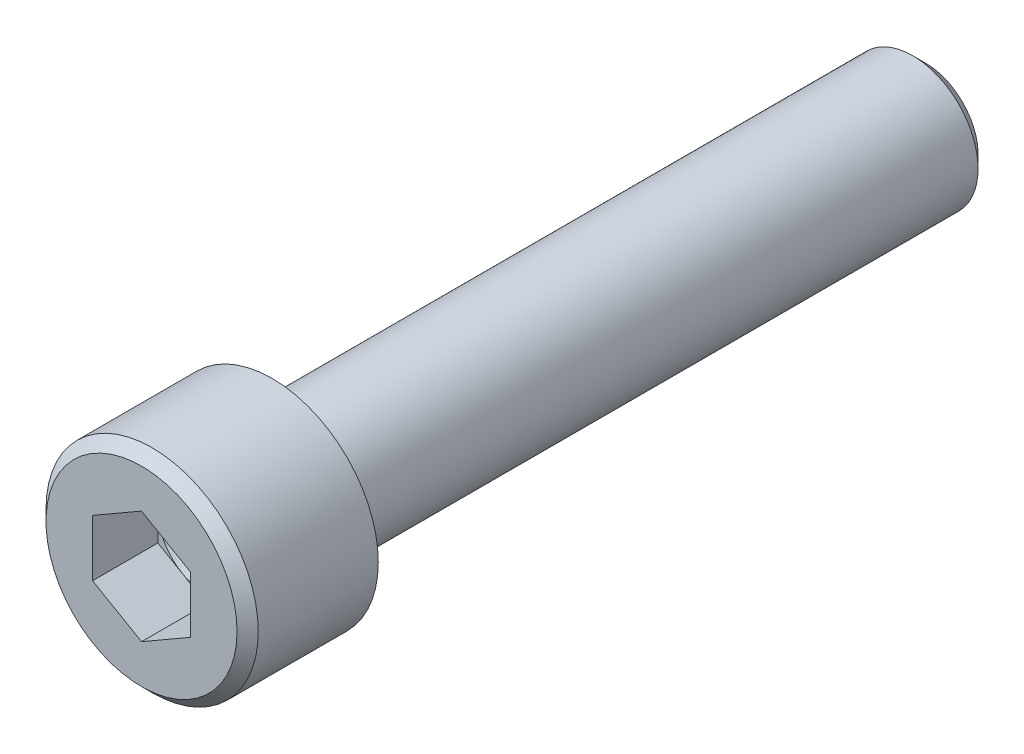
from build123d import *

# Parameters (mm, degrees)
SKETCH_1_W          = 6.5
SKETCH_1_H          = 8
SKETCH_2_R          = 4
EXTRUDE_1_DEPTH     = 40
CUT_EXTRUDE_1_DEPTH = 4
CHAMFER_1_SIZE      = 0.65
CHAMFER_2_SIZE      = 0.767


with BuildPart() as part:
    # 草图1 → 旋转1 (revolve)
    with BuildSketch(Plane(origin=(0, 0, 0), x_dir=(1, 0, 0), z_dir=(0, 1, 0))):
        with Locations((3.25, -4)):
            Rectangle(SKETCH_1_W, SKETCH_1_H)
    revolve(axis=Axis((0, 0, 0), (0, 0, 1)))

    # 草图2 → 凸台-拉伸1 (add)
    with BuildSketch(Plane(origin=(0, 0, 0), x_dir=(-1, 0, 0), z_dir=(0, 0, -1))):
        Circle(SKETCH_2_R)
    extrude(amount=EXTRUDE_1_DEPTH)

    # 草图3 → 切除-拉伸1 (cut)
    with BuildSketch(Plane.XY.offset(8)):
        Polygon((3, 1.732050808), (0, 3.464101615), (-3, 1.732050808), (-3, -1.732050808), (0, -3.464101615), (3, -1.732050808), align=None)
    extrude(amount=-CUT_EXTRUDE_1_DEPTH, mode=Mode.SUBTRACT)

    # 草图4 → 切除-旋转1 (revolve, cut)
    with BuildSketch(Plane.XZ, mode=Mode.PRIVATE) as cut_revolve_1_sk:
        Polygon((3, 4), (0, 4), (0, 2.267949192), align=None)
    revolve(cut_revolve_1_sk.sketch.rotate(Axis((0, 0, 4), (0, 0, -1)), 90), axis=Axis((0, 0, 4), (0, 0, -1)), mode=Mode.SUBTRACT)

    # 倒角1
    chamfer_1_edges = [part.edges().sort_by_distance(p)[0] for p in [
        (-6.5, 0, 8),
    ]]
    chamfer(chamfer_1_edges, length=CHAMFER_1_SIZE)

    # 倒角2
    chamfer_2_edges = [part.edges().sort_by_distance(p)[0] for p in [
        (4, 0, -40),
    ]]
    chamfer(chamfer_2_edges, length=CHAMFER_2_SIZE)


solid = part.part
